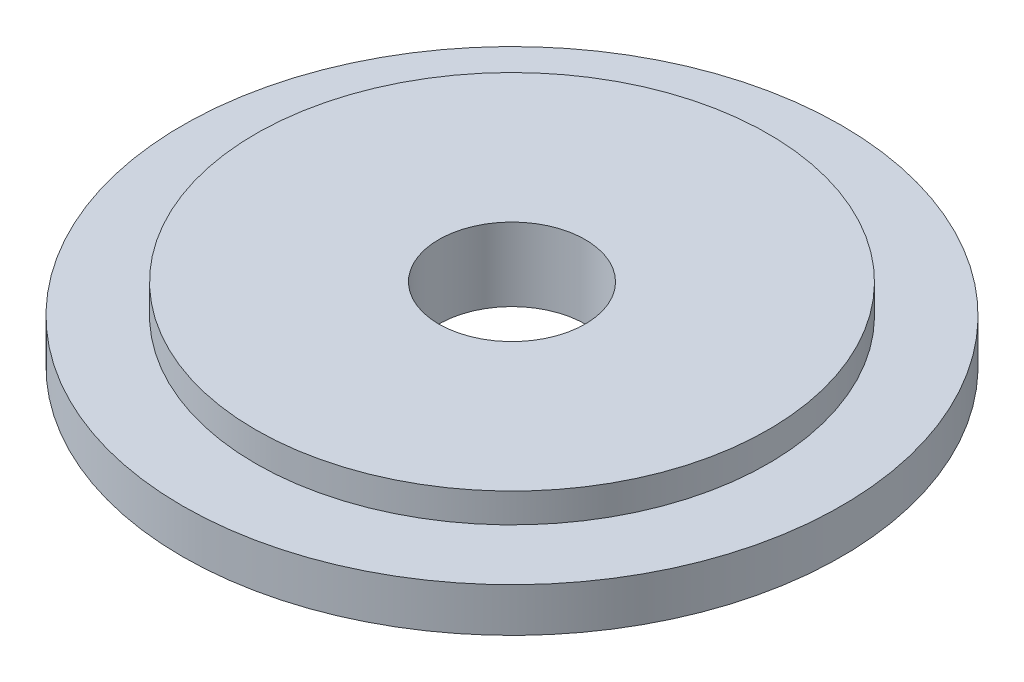
from build123d import *

# Parameters (mm, degrees)
SKETCH_1_R          = 22.5
EXTRUDE_1_DEPTH     = 3
SKETCH_2_R          = 17.5
EXTRUDE_2_DEPTH     = 2
SKETCH_3_R          = 5
CUT_EXTRUDE_1_DEPTH = 33.210246817


with BuildPart() as part:
    # 草图1 → 凸台-拉伸1 (new body)
    with BuildSketch(Plane(origin=(0, 0, 0), x_dir=(1, 0, 0), z_dir=(0, 1, 0))):
        with Locations(Location((0, 0, 0), (0, 0, 270))):
            Circle(SKETCH_1_R)
    extrude(amount=EXTRUDE_1_DEPTH)

    # 草图2 → 凸台-拉伸2 (add)
    with BuildSketch(Plane(origin=(0, 3, 0), x_dir=(1, 0, 0), z_dir=(0, 1, 0))):
        with Locations(Location((0, 0, 0), (0, 0, 270))):
            Circle(SKETCH_2_R)
    extrude(amount=EXTRUDE_2_DEPTH)

    # 草图3 → 切除-拉伸1 (cut, through all)
    with BuildSketch(Plane(origin=(0, 5, 0), x_dir=(1, 0, 0), z_dir=(0, 1, 0))):
        with Locations(Location((0, 0, 0), (0, 0, 270))):
            Circle(SKETCH_3_R)
    extrude(amount=-CUT_EXTRUDE_1_DEPTH, mode=Mode.SUBTRACT)


solid = part.part
